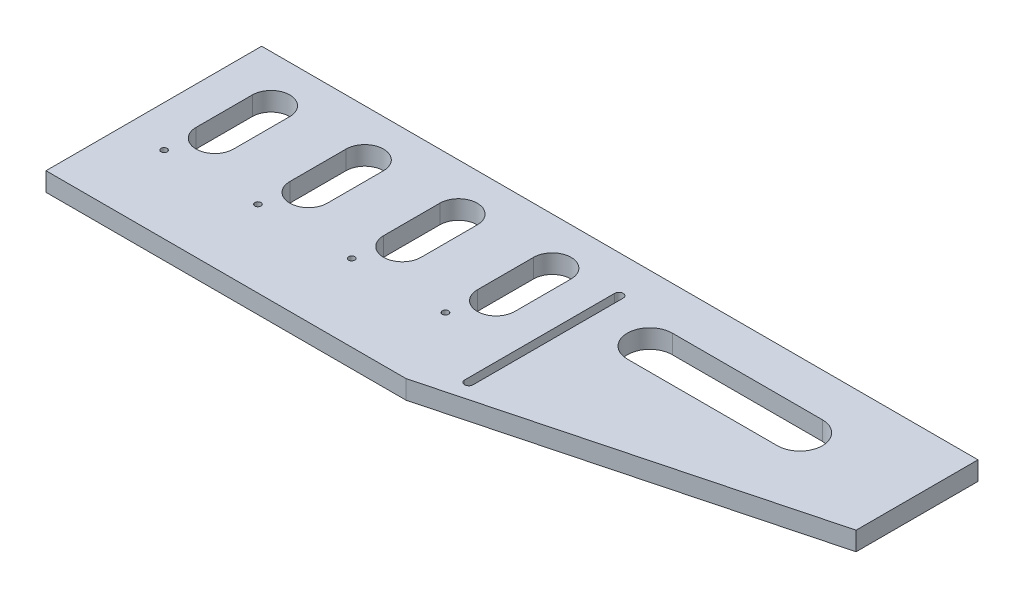
SolidWorks part; units mm, degrees
material "AL6061"
ref_plane "前视" through (0, 0, 0) normal (0, 0, 1) x (1, 0, 0)
ref_plane "上视" through (0, 0, 0) normal (0, 1, 0) x (1, 0, 0)
ref_plane "右视" through (0, 0, 0) normal (1, 0, 0) x (0, 0, -1)
sketch "草图1" plane through (0, 0, 0) normal (0, 1, 0) x (1, 0, 0)
  line L1 (-191, 40) -> (191, 40)
  line L2 (-191, 40) -> (-191, -40)
  line L3 (-191, -40) -> (191, -40)
  line L4 (191, 40) -> (191, -40)
  line L5 (-191, 40) -> (191, -40) construction
  line L6 (-191, -40) -> (191, 40) construction
  point P0 (0, 0)
  dimension "D1" = 382
  dimension "D2" = 80
extrude "凸台-拉伸1" add sketch "草图1" along normal blind 10
hole_wizard "M3 螺纹孔1" positions "草图2" profile "草图3" tap size "M3" standard "GB"
sketch "草图2" plane through (0, 0, -40) normal (0, 0, -1) x (-1, 0, 0)
  line L0 (191, 10) -> (191, 0) construction
  point P0 (187, 5)
  point P5 (-187, 5)
  point P9 (191, 5)
  dimension "D1" = 4
  dimension "D2" = 374
sketch "草图3" plane through (-187, 5, -40) normal (1, 0, 0) x (0, 1, 0)
  line L0 (0, 0) -> (0, 9.2511)
  line L1 (0, 9.2511) -> (1.25, 8.5)
  line L2 (1.25, 8.5) -> (1.25, 0)
  line L5 (1.25, 0) -> (0, 0)
  line L10 (0, 9.2511) -> (-1.25, 8.5) construction
  line L11 (0, -6.35) -> (0, 107.95) construction
  dimension "螺纹孔钻头直径" = 2.5
  dimension "螺纹孔钻头深度" = 8.5
  dimension "导头角度" = 118
cosmetic thread "孔螺蚊线2" parameters "D1"=6, "D2"=3
cosmetic thread "孔螺蚊线6" parameters "D1"=6, "D2"=3
sketch "草图4" plane through (0, 10, 0) normal (0, 1, 0) x (1, 0, 0)
  line L0 (-11, 15) -> (-11, -15) construction
  line L1 (-1, 15) -> (-1, -15)
  line L2 (-21, 15) -> (-21, -15)
  line L3 (-191, 40) -> (-191, -40) construction
  arc A0 (-1, 15) -> (-21, 15) centre (-11, 15) ccw
  arc A1 (-21, -15) -> (-1, -15) centre (-11, -15) ccw
  point P2 (-11, 0)
  point P10 (-191, 0)
  dimension "D1" = 10
  dimension "D2" = 30
  dimension "D3" = 180
extrude "切除-拉伸1" cut sketch "草图4" against normal through all
pattern_linear "阵列(线性)1" count 4 spacing 50 along (-1, 0, 0) of "切除-拉伸1"
sketch "草图6" plane through (0, 10, 0) normal (0, 1, 0) x (1, 0, 0)
  circle A2 centre (19.5, -31.4773) radius 1.65
  circle A3 centre (19.5, -11.4773) radius 1.65
hole_wizard "M4 间隙孔1" positions "草图7" profile "草图8" hole size "M4" standard "ISO" end condition through all
sketch "草图7" plane through (0, 10, 0) normal (0, 1, 0) x (1, 0, 0)
  line L0 (-191, 40) -> (-191, -40) construction
  line L1 (-191, -40) -> (191, -40) construction
  point P0 (19.5, -11)
  point P2 (19.5, -31)
  dimension "D1" = 20
  dimension "D2" = 210.5
  dimension "D3" = 29
  dimension "D4" = 0
sketch "草图8" plane through (19.5, 10, 11) normal (1, 0, 0) x (0, 0, 1)
  line L0 (0, 0) -> (0, 10)
  line L1 (0, 10) -> (2.25, 10)
  line L2 (2.25, 10) -> (2.25, 0)
  line L5 (2.25, 0) -> (0, 0)
  line L11 (0, -6.35) -> (0, 107.95) construction
  dimension "通孔孔直径" = 4.5
  dimension "通孔孔深度" = 10
hole_wizard "M4 螺纹孔1" positions "草图9" profile "草图10" tap size "M4" standard "ISO" end condition through all
sketch "草图9" plane through (0, 10, 0) normal (0, 1, 0) x (1, 0, 0)
  line L0 (-191, -40) -> (191, -40) construction
  line L1 (191, -40) -> (191, 40) construction
  point P0 (-19, -34)
  dimension "D1" = 6
  dimension "D2" = 210
sketch "草图10" plane through (-19, 10, 34) normal (1, 0, 0) x (0, 0, 1)
  line L0 (0, 0) -> (0, 10)
  line L1 (0, 10) -> (1.65, 10)
  line L2 (1.65, 10) -> (1.65, 0)
  line L5 (1.65, 0) -> (0, 0)
  line L11 (0, -6.35) -> (0, 107.95) construction
  dimension "通孔螺纹孔钻头直径" = 3.3
  dimension "通孔螺纹孔钻头深度" = 10
cosmetic thread "孔螺蚊线3" parameters "D2"=4
pattern_linear "阵列(线性)2" count 4 spacing 50 along (-1, 0, 0) of "M4 螺纹孔1"
hole_wizard "M4 螺纹孔2" positions "草图11" profile "草图12" tap size "M4" standard "ISO"
sketch "草图11" plane through (-191, 0, 0) normal (-1, 0, 0) x (0, 0, 1)
  line L0 (40, 10) -> (40, 0) construction
  line L1 (-27.5, 5) -> (27.5, 5) construction
  line L3 (-40, 0) -> (40, 0) construction
  point P0 (27.5, 5)
  point P2 (-27.5, 5)
  point P6 (40, 5)
  point P10 (0, 5)
  point P13 (0, 0)
  dimension "D1" = 55
sketch "草图12" plane through (-191, 5, 27.5) normal (0, 1, 0) x (0, 0, 1)
  line L0 (0, 0) -> (0, 11.0914)
  line L1 (0, 11.0914) -> (1.65, 10.1)
  line L2 (1.65, 10.1) -> (1.65, 0)
  line L5 (1.65, 0) -> (0, 0)
  line L10 (0, 11.0914) -> (-1.65, 10.1) construction
  line L11 (0, -6.35) -> (0, 107.95) construction
  dimension "螺纹孔钻头直径" = 3.3
  dimension "螺纹孔钻头深度" = 10.1
  dimension "导头角度" = 118
cosmetic thread "孔螺蚊线4" parameters "D1"=8, "D2"=4
cosmetic thread "孔螺蚊线5" parameters "D1"=8, "D2"=4
sketch "草图14" plane through (0, 0, 0) normal (0, -1, 0) x (1, 0, 0)
  line L0 (19.5, 33.25) -> (19.5, 28.75) construction
  line L1 (21.75, 33.25) -> (21.75, 28.75)
  line L2 (17.25, 33.25) -> (17.25, 28.75)
  line L3 (19.5, 13.25) -> (19.5, 8.75) construction
  line L4 (21.75, 13.25) -> (21.75, 8.75)
  line L5 (17.25, 13.25) -> (17.25, 8.75)
  circle A0 centre (19.5, 31) radius 2.25 construction
  arc A1 (21.75, 33.25) -> (17.25, 33.25) centre (19.5, 33.25) ccw
  arc A2 (17.25, 28.75) -> (21.75, 28.75) centre (19.5, 28.75) ccw
  circle A3 centre (19.5, 11) radius 2.25 construction
  arc A4 (21.75, 13.25) -> (17.25, 13.25) centre (19.5, 13.25) ccw
  arc A5 (17.25, 8.75) -> (21.75, 8.75) centre (19.5, 8.75) ccw
  point P4 (19.5, 31)
  point P9 (19.5, 11)
  dimension "D1" = 4.5
  dimension "D2" = 4.5
extrude "切除-拉伸3" cut sketch "草图14" against normal blind 10
other "移动面1" face at (0, 5, 40) parameters "D1"=35
sketch "草图15" plane through (0, 0, 0) normal (0, -1, 0) x (1, 0, 0)
  line L0 (19.5, 60) -> (19.5, -20) construction
  line L1 (21.75, 60) -> (21.75, -20)
  line L2 (17.25, 60) -> (17.25, -20)
  line L3 (21.75, 28.75) -> (21.75, 33.25) construction
  line L4 (17.25, 33.25) -> (17.25, 28.75) construction
  line L5 (191, -40) -> (-191, -40) construction
  arc A0 (21.75, 60) -> (17.25, 60) centre (19.5, 60) ccw
  arc A1 (17.25, -20) -> (21.75, -20) centre (19.5, -20) ccw
  point P2 (19.5, 20)
  dimension "D1" = 20
  dimension "D2" = 80
extrude "切除-拉伸4" cut sketch "草图15" against normal through all
chamfer "倒角1" distance 190 distance2 50 1 edges at (191, 5, 75)
sketch "草图5" plane through (0, 10, 0) normal (0, 1, 0) x (1, 0, 0)
  line L0 (131, 5) -> (51, 5) construction
  line L1 (131, -7) -> (51, -7)
  line L2 (131, 17) -> (51, 17)
  line L3 (191, 40) -> (-191, 40) construction
  line L4 (191, -25) -> (191, 40) construction
  arc A0 (131, -7) -> (131, 17) centre (131, 5) ccw
  arc A1 (51, 17) -> (51, -7) centre (51, 5) ccw
  point P2 (91, 5)
  dimension "D1" = 12
  dimension "D2" = 35
  dimension "D3" = 80
  dimension "D4" = 60
extrude "切除-拉伸2" cut sketch "草图5" against normal through all
